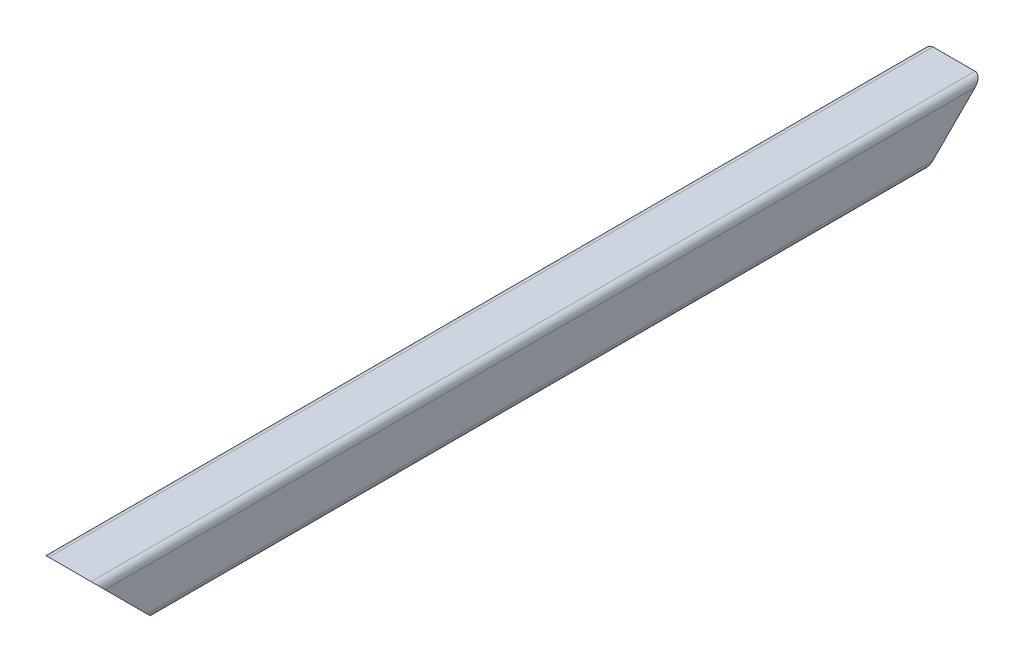
SolidWorks part; units mm, degrees
ref_plane "Front Plane" through (0, 0, 0) normal (0, 0, 1) x (1, 0, 0)
ref_plane "Top Plane" through (0, 0, 0) normal (0, 1, 0) x (1, 0, 0)
ref_plane "Right Plane" through (0, 0, 0) normal (1, 0, 0) x (0, 0, -1)
sketch "Sketch 1" plane through (0, 0, 0) normal (0, 0, 1) x (1, 0, 0)
  line L0 (0, 96.8978) -> (0, -107.4818) construction
  line L1 (-129.1971, 0) -> (137.9562, 0) construction
  line L2 (0, 32) -> (-24, 32)
  line L3 (-32, 24) -> (-32, 0)
  line L4 (0, 28) -> (-24, 28)
  line L5 (-28, 24) -> (-28, 0)
  line L6 (-28, -24) -> (-28, 0)
  line L7 (24, -28) -> (-24, -28)
  line L8 (-32, -24) -> (-32, 0)
  line L9 (24, -32) -> (-24, -32)
  line L10 (32, -24) -> (32, 0)
  line L11 (28, -24) -> (28, 0)
  line L12 (28, 24) -> (28, 0)
  line L13 (0, 28) -> (24, 28)
  line L14 (32, 24) -> (32, 0)
  line L15 (0, 32) -> (24, 32)
  arc A0 (-24, 32) -> (-32, 24) centre (-24, 24) ccw
  arc A1 (-24, 28) -> (-28, 24) centre (-24, 24) ccw
  arc A2 (-24, -28) -> (-28, -24) centre (-24, -24) cw
  arc A3 (-24, -32) -> (-32, -24) centre (-24, -24) cw
  arc A4 (24, -32) -> (32, -24) centre (24, -24) ccw
  arc A5 (24, -28) -> (28, -24) centre (24, -24) ccw
  arc A6 (24, 28) -> (28, 24) centre (24, 24) cw
  arc A7 (24, 32) -> (32, 24) centre (24, 24) cw
  point P34 (0, -32)
  point P35 (0, -28)
  dimension "D3" = 8
  dimension "D1" = 64
  dimension "D2" = 64
  dimension "D4" = 4
extrude "Boss-Extrude 1" add sketch "Sketch 1" along normal mid plane 1006.76
sketch "Sketch 2" plane through (0, 0, 0) normal (1, 0, 0) x (0, 0, -1)
  line L0 (0, 50.6454) -> (0, -55.4996) construction
  line L1 (-503.38, 32) -> (-439.38, -32)
  line L2 (-503.38, -32) -> (503.38, -32) construction
  line L3 (-439.38, -32) -> (-503.38, -32)
  line L4 (-503.38, -32) -> (-503.38, 32)
  line L5 (503.38, -32) -> (503.38, 32)
  line L6 (439.38, -32) -> (503.38, -32)
  line L7 (503.38, 32) -> (439.38, -32)
extrude "Cut-Extrude 1" cut sketch "Sketch 2" against normal through all both and the other way through all
